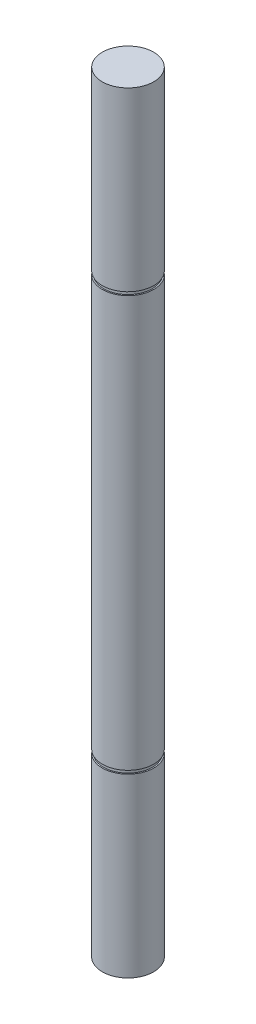
SolidWorks part; units mm, degrees
ref_plane "前视基准面" through (0, 0, 0) normal (0, 0, 1) x (1, 0, 0)
ref_plane "上视基准面" through (0, 0, 0) normal (0, 1, 0) x (1, 0, 0)
ref_plane "右视基准面" through (0, 0, 0) normal (1, 0, 0) x (0, 0, -1)
sketch "草图1" plane through (0, 0, 0) normal (0, 1, 0) x (1, 0, 0)
  circle A0 centre (0, 0) radius 10
  dimension "D1" = 20
extrude "凸台-拉伸1" add sketch "草图1" along normal blind 300
ref_plane "基准面1" through (0, 0, -10) normal (0, 0, -1) x (-1, 0, 0)
ref_plane "基准面3" through (0, 70, 0) normal (0, -1, 0) x (-1, 0, 0)
sketch "草图7" plane through (0, 70, 0) normal (0, -1, 0) x (-1, 0, 0)
  circle A0 centre (0, 0) radius 10 construction
  circle A1 centre (0, 0) radius 10
  circle A2 centre (0, 0) radius 9.5
  dimension "D1" = 19
extrude "切除-拉伸3" cut sketch "草图7" along normal blind 1.3
ref_plane "基准面4" through (0, 230, 0) normal (0, 1, 0) x (1, 0, 0)
sketch "草图8" plane through (0, 230, 0) normal (0, 1, 0) x (1, 0, 0)
  circle A0 centre (0, 0) radius 10 construction
  circle A1 centre (0, 0) radius 10
  circle A2 centre (0, 0) radius 9.5
  dimension "D1" = 19
extrude "切除-拉伸4" cut sketch "草图8" along normal blind 1.3
chamfer "倒角1" [suppressed] distance 0.5 angle 45
ref_plane "基准面2" through (0, 65, 0) normal (0, -1, 0) x (-1, 0, 0)
sketch "MyToolsJD" plane through (0, 0, 0) normal (0, -1, 0) x (-1, 0, 0)
  line L0 (0, 0) -> (10, 0) construction
  line L1 (0, 0) -> (0, 10) construction
  circle A0 centre (0, 0) radius 10 construction
  circle A1 centre (0, 0) radius 10 construction
  dimension "D1" = 90
ref_plane "基准面11" through (0, 0, -10) normal (0, 0, -1) x (-1, 0, 0)
sketch "MyToolsZJC" plane through (0, 0, -10) normal (0, 0, -1) x (0, 1, 0)
  line L0 (148, 0) -> (152, 0) construction
  line L1 (148, 3) -> (152, 3)
  line L2 (148, -3) -> (152, -3)
  line L3 (0, 0) -> (148, 0) construction
  line L5 (150, 10) -> (150, -35.6075) construction
  line L6 (230, 10) -> (70, 10) construction
  arc A0 (148, 3) -> (148, -3) centre (148, 0) ccw
  arc A1 (152, -3) -> (152, 3) centre (152, 0) ccw
  point P2 (150, 0)
  point P13 (155, 0)
  point P14 (145, 0)
  dimension "D3" = 10
  dimension "D1" = 6
extrude "ZJCQC" cut sketch "MyToolsZJC" against normal blind 3.5
